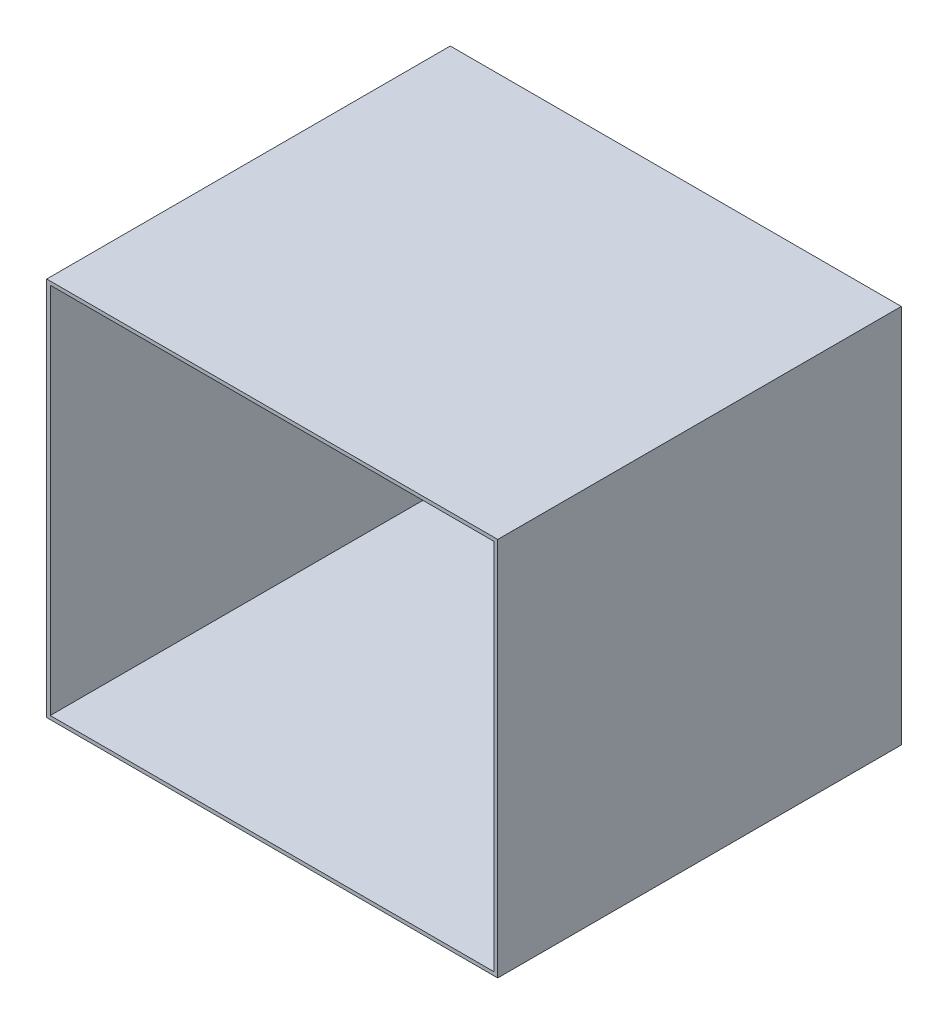
SolidWorks part; units mm, degrees
ref_plane "前视基准面" through (0, 0, 0) normal (0, 0, 1) x (1, 0, 0)
ref_plane "上视基准面" through (0, 0, 0) normal (0, 1, 0) x (1, 0, 0)
ref_plane "右视基准面" through (0, 0, 0) normal (1, 0, 0) x (0, 0, -1)
other "Configuration Table"
sketch "草图1" plane through (0, 0, 0) normal (0, 0, 1) x (1, 0, 0)
  line L0 (-190, -160) -> (190, -160)
  line L1 (190, -160) -> (190, 160)
  line L2 (190, 160) -> (-190, 160)
  line L3 (-190, 160) -> (-190, -160)
  line L4 (-187, -157) -> (187, -157)
  line L5 (187, -157) -> (187, 157)
  line L6 (187, 157) -> (-187, 157)
  line L7 (-187, 157) -> (-187, -157)
  point P0 (0, 0)
  dimension "D1" = 3
  dimension "D2" = 190
  dimension "D3" = 377
  dimension "D4" = 380
  dimension "D5" = 3
  dimension "D6" = 160
  dimension "D7" = 317
  dimension "D8" = 320
extrude "凸台-拉伸1" add sketch "草图1" against normal mid plane 340
